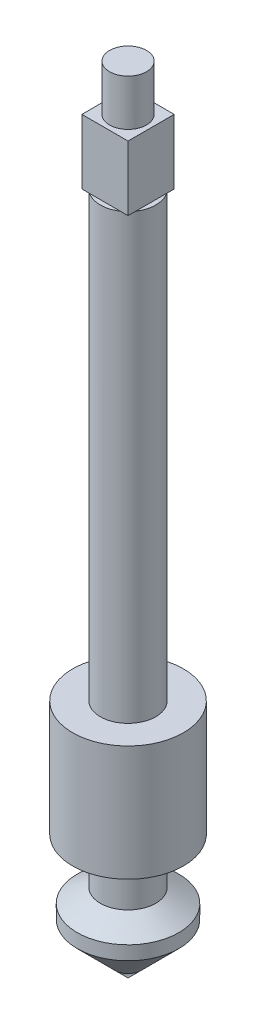
from build123d import *

# Parameters (mm, degrees)
SKETCH2_W           = 10
SKETCH2_H           = 10
BOSS_EXTRUDE1_DEPTH = 14
SKETCH3_R           = 4
BOSS_EXTRUDE2_DEPTH = 10


with BuildPart() as part:
    # Sketch1 → Revolve1 (revolve)
    with BuildSketch(Plane.XY, mode=Mode.PRIVATE) as revolve1_sk:
        Polygon((0, 0), (-11, 11), (-11, 14), (-6, 17), (-6, 27), (-12, 27), (-12, 52), (-6, 52), (-6, 148), (0, 148), align=None)
    revolve(revolve1_sk.sketch.rotate(Axis((0, -1000, 0), (0, 1, 0)), 180), axis=Axis((0, -1000, 0), (0, 1, 0)))

    # Sketch2 → Boss-Extrude1 (add)
    with BuildSketch(Plane(origin=(0, 148, 0), x_dir=(1, 0, 0), z_dir=(0, 1, 0))):
        Rectangle(SKETCH2_W, SKETCH2_H)
    extrude(amount=BOSS_EXTRUDE1_DEPTH)

    # Sketch3 → Boss-Extrude2 (add)
    with BuildSketch(Plane(origin=(0, 162, 0), x_dir=(1, 0, 0), z_dir=(0, 1, 0))):
        Circle(SKETCH3_R)
    extrude(amount=BOSS_EXTRUDE2_DEPTH)


solid = part.part
